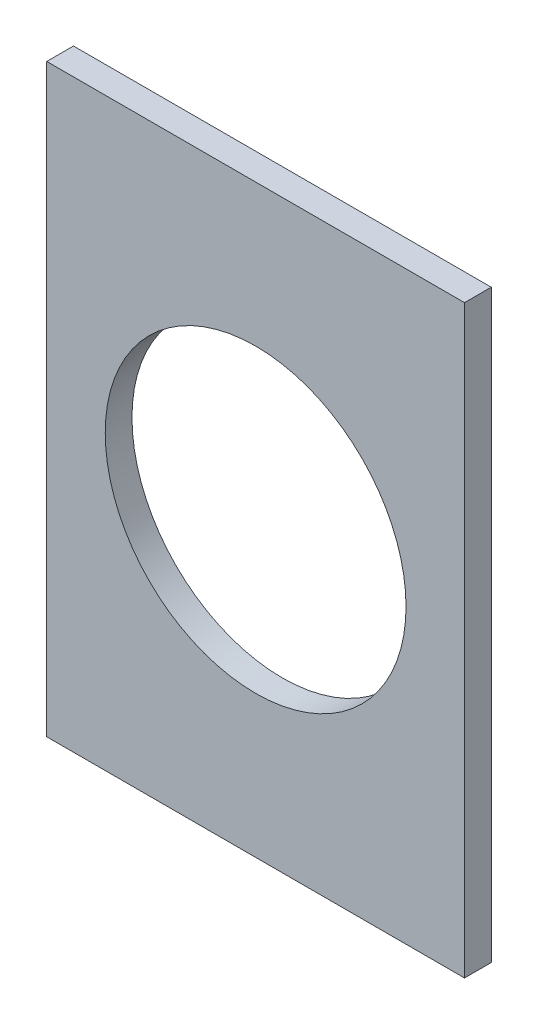
SolidWorks part; units mm, degrees
material "XRAAT"
ref_plane "前视基准面" through (0, 0, 0) normal (0, 0, 1) x (1, 0, 0)
ref_plane "上视基准面" through (0, 0, 0) normal (0, 1, 0) x (1, 0, 0)
ref_plane "右视基准面" through (0, 0, 0) normal (1, 0, 0) x (0, 0, -1)
sketch "草图1" plane through (0, 0, 0) normal (0, 0, 1) x (1, 0, 0)
  line L1 (125, -175) -> (-125, -175)
  line L2 (125, -175) -> (125, 175)
  line L3 (125, 175) -> (-125, 175)
  line L4 (-125, -175) -> (-125, 175)
  line L5 (125, -175) -> (-125, 175) construction
  line L6 (125, 175) -> (-125, -175) construction
  circle A0 centre (0, 0) radius 90
  point P0 (0, 0)
  dimension "D3" = 180
  dimension "D1" = 350
  dimension "D2" = 250
extrude "凸台-拉伸1" add sketch "草图1" along normal blind 16
